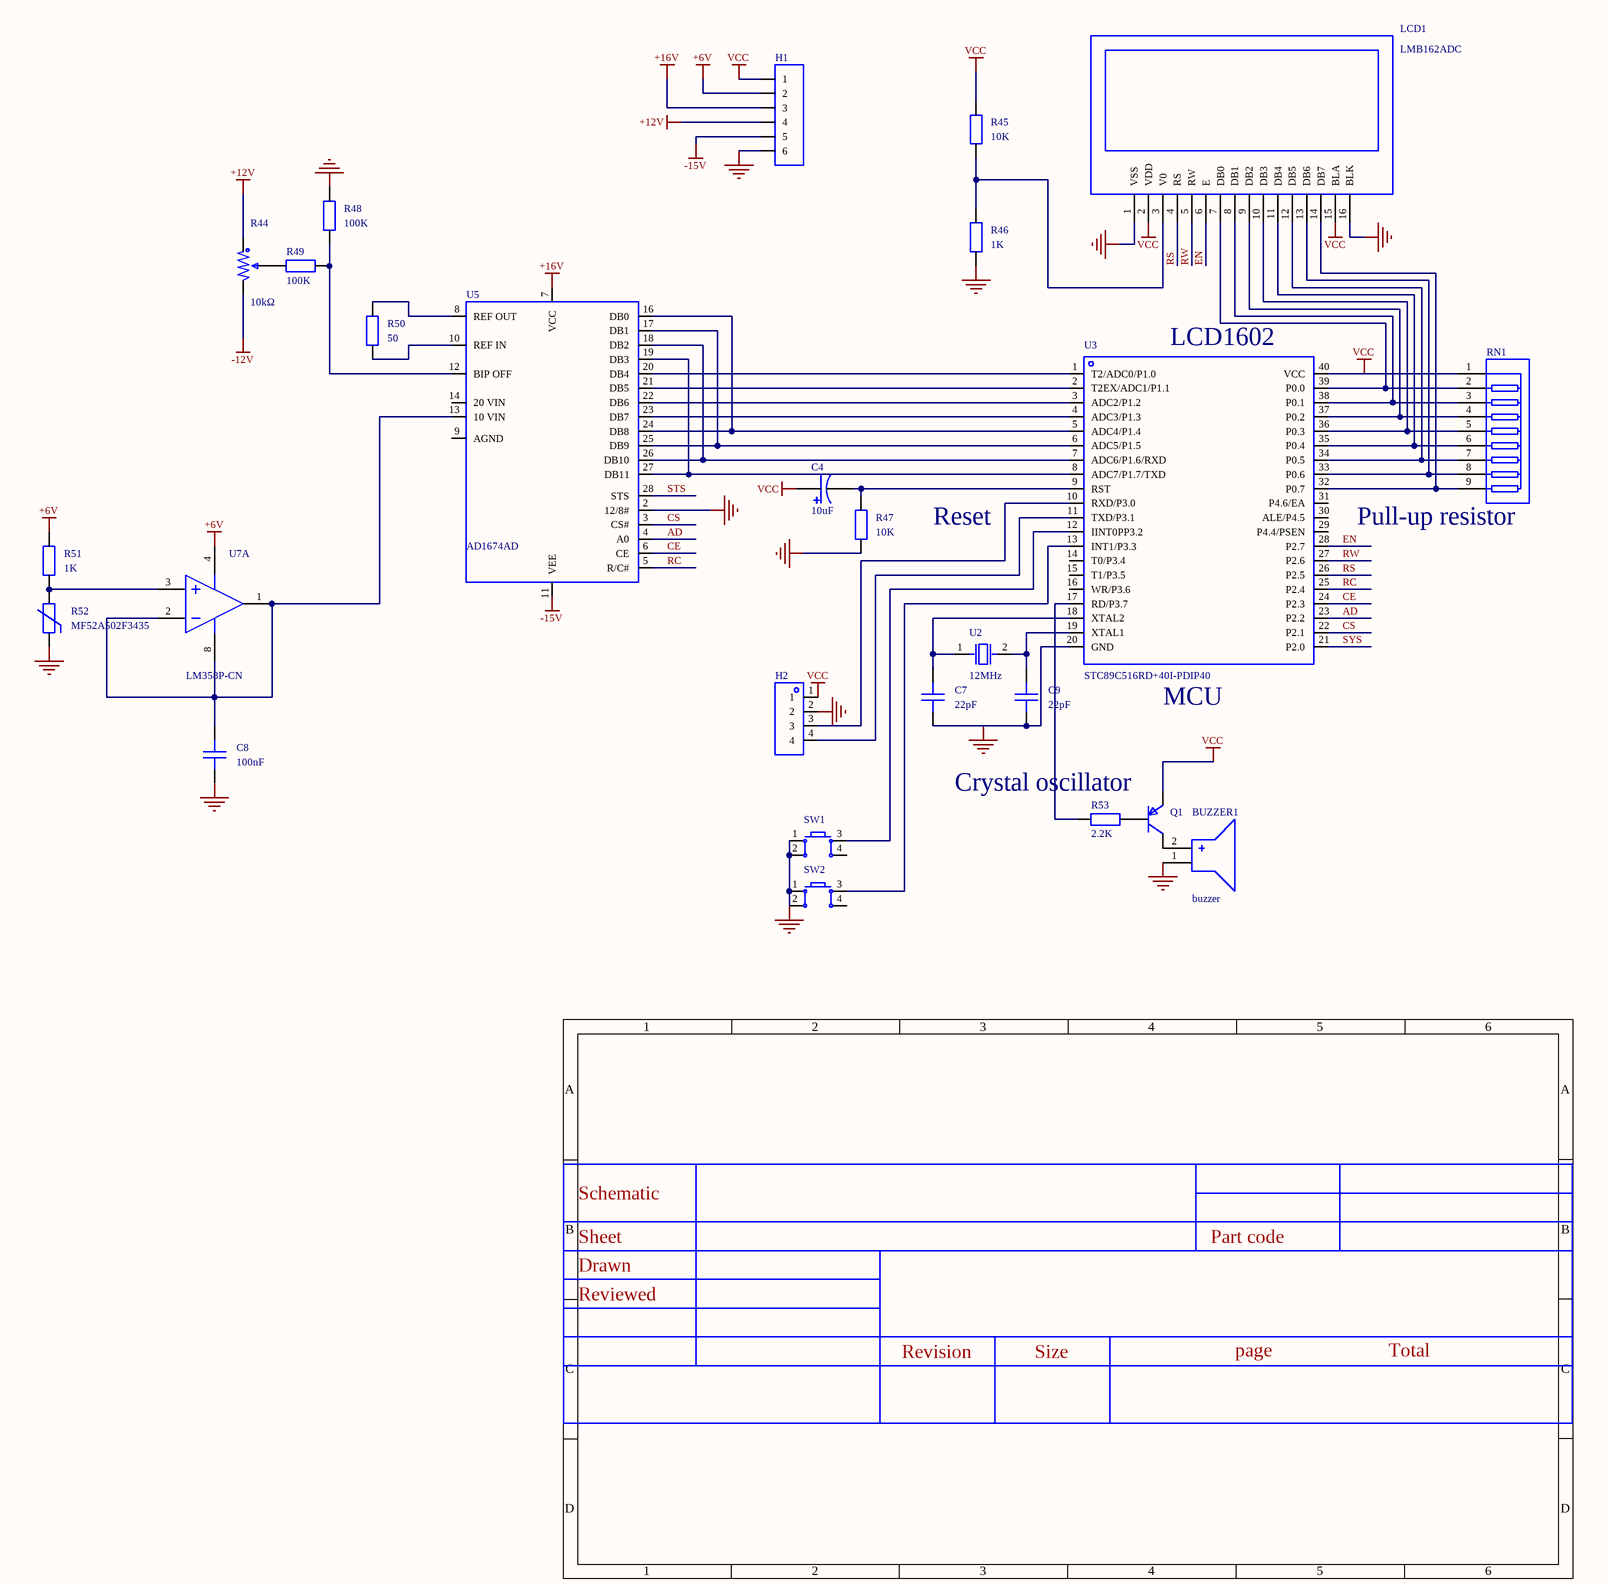
[diagram p0: MISC51839-3.schdoc]
# Altium project MISC51839-2.PrjPcb
1 sheet, 26 parts. Net scope: global (net labels, ports and power ports of the same name join across sheets).
Board file: MISC51839.pcbdoc

## Sheet MISC51839-3.schdoc
size 178 x 98 mm; Version: V1.0; @Project Name: MISC51839; @Page Count: 1; @Update Date: 2025-05-19; @Create Date: 2025-05-19; @Schematic Name: MISC51839; @Page No: 1; @Board Name: MISC51839; @Create Time: 08:04:37; @Update Time: 08:33:31

### Parts
BUZZER1  buzzer  [BUZ-TH_BD12.0-P6.00-D0.9-RD]
C4  10uF  [CAP-TH_BD6.3-P2.50-D1.0-FD]
C7  22pF  [C0603]
C8  100nF  [C0805]
C9  22pF  [C0603]
H1  (no value)  [HDR-TH_6P-P2.54-V-M-1]
H2  (no value)  [HDR-TH_4P-P2.54-V-F]
LCD1  LMB162ADC  [LCD1602]
Q1  (no value)  [S8550P_SOT]
R44  10kΩ  [RES-ADJ-SMD_RM065-V1]
R45  10K  [R0603]
R46  1K  [R0603]
R47  10K  [R0603]
R48  100K  [R0603]
R49  100K  [R0603]
R50  50  [R0603]
R51  1K  [R0603]
R52  MF52A502F3435  [RES-TH_BD2.0-P1.80-D0.3]
R53  2.2K  [R0603]
RN1  -  [RES-ARRAY-TH_9P-P2.54-D1.0]
SW1  (no value)  [SW-TH_4P-L6.0-W6.0-P4.50-LS6.5]
SW2  (no value)  [SW-TH_4P-L6.0-W6.0-P4.50-LS6.5]
U2  12MHz  [HC-49US_L11.0-W4.6-P4.88]
U3  STC89C516RD+40I-PDIP40  [DIP-40_L52.3-W13.9-P2.54-LS15.2-BL]
U5  AD1674AD  [CDIP-28_L35.5-W14.8-P2.54-LS15.3-BL]
U7  LM358P-CN  [SOIC-8_L5.0-W4.0-P1.27-LS6.0-BL]  (part A of 2)

### Nets
+6V: H1.2 R51.2 U7.4(V-)
+12V: H1.4 R44.1
+16V: H1.3 U5.7(VCC)
-12V: R44.3
-15V: H1.5 U5.11(VEE)
GND: BUZZER1.1(-) C7.1 C8.1 C9.1 H1.6 H2.2 LCD1.1(VSS) LCD1.16(BLK) R46.1 R47.1 R48.2 R52.1 SW1.1 SW1.2 SW2.1 SW2.2 U3.20(GND) U5.2(12/8#)
VCC: C4.1 H1.1 H2.1 LCD1.2(VDD) LCD1.15(BLA) Q1.2(E) R45.2 RN1.1 U3.40(VCC)
AD: U3.23(P2.2) U5.4(A0)
CE: U3.24(P2.3) U5.6(CE)
CS: U3.22(P2.1) U5.3(CS#)
EN: LCD1.6(E) U3.28(P2.7)
RC: U3.25(P2.4) U5.5(R/C#)
RS: LCD1.4(RS) U3.26(P2.5)
RW: LCD1.5(RW) U3.27(P2.6)
STS: U5.28(STS)
SYS: U3.21(P2.0)
NetBUZZER1_2: BUZZER1.2(+) Q1.3(C)
NetC4_2: C4.2 R47.2 U3.9(RST)
NetC7_2: C7.2 U2.1(OSC1) U3.18(XTAL2)
NetC8_2: C8.2 U5.13(10_VIN) U7.1(OUT1) U7.2(IN1-) U7.8(V+)
NetC9_2: C9.2 U2.2(OSC2) U3.19(XTAL1)
NetH2_3: H2.3 U3.10(RXD/P3.0)
NetH2_4: H2.4 U3.11(TXD/P3.1)
NetLCD1_3: LCD1.3(V0) R45.1 R46.2
NetLCD1_7: LCD1.7(DB0) RN1.2 U3.39(P0.0)
NetLCD1_8: LCD1.8(DB1) RN1.3 U3.38(P0.1)
NetLCD1_9: LCD1.9(DB2) RN1.4 U3.37(P0.2)
NetLCD1_10: LCD1.10(DB3) RN1.5 U3.36(P0.3)
NetLCD1_11: LCD1.11(DB4) RN1.6 U3.35(P0.4)
NetLCD1_12: LCD1.12(DB5) RN1.7 U3.34(P0.5)
NetLCD1_13: LCD1.13(DB6) RN1.8 U3.33(P0.6)
NetLCD1_14: LCD1.14(DB7) RN1.9 U3.32(P0.7)
NetQ1_1: Q1.1(B) R53.2
NetR44_2: R44.2 R49.2
NetR48_1: R48.1 R49.1 U5.12(BIP_OFF)
NetR50_1: R50.1 U5.10(REF_IN)
NetR50_2: R50.2 U5.8(REF_OUT)
NetR51_1: R51.1 R52.2 U7.3(IN1+)
NetR53_1: R53.1 U3.17(RD/P3.7)
NetSW1_3: SW1.3 U3.12(IINT0PP3.2)
NetSW2_3: SW2.3 U3.13(INT1/P3.3)
NetU3_1: U3.1(T2/ADC0/P1.0) U5.20(DB4)
NetU3_2: U3.2(T2EX/ADC1/P1.1) U5.21(DB5)
NetU3_3: U3.3(ADC2/P1.2) U5.22(DB6)
NetU3_4: U3.4(ADC3/P1.3) U5.23(DB7)
NetU3_5: U3.5(ADC4/P1.4) U5.16(DB0) U5.24(DB8)
NetU3_6: U3.6(ADC5/P1.5) U5.17(DB1) U5.25(DB9)
NetU3_7: U3.7(ADC6/P1.6/RXD) U5.18(DB2) U5.26(DB10)
NetU3_8: U3.8(ADC7/P1.7/TXD) U5.19(DB3) U5.27(DB11)

Not connected (* = marked no-connect by the designer): SW1 4; SW2 4; U3 14(T0/P3.4) 15(T1/P3.5) 16(WR/P3.6) 29(P4.4/PSEN) 30(ALE/P4.5) 31(P4.6/EA); U5 9(AGND) 14(20_VIN)

### Notes on the sheet
- (near U3) LCD1602
- Reset
- (near RN1) Pull-up resistor
- (near U3) MCU
- (near Q1) Crystal oscillator
- 2025-05-19
- Schematic
- Sheet
- Part code
- P1
- Reviewed
- Drawn
- Revision
- Size
- page
- Total
- A4
- 1

### Library data of the parts
BUZZER1 = buzzer: AddInBom: yes; ModelId: af17e4151ed84fc2a628230bf2376363; ModelTransform: 472.44,472.176,0,270,0,0,0,0,-196.85; Symbol: BUZZER; Device: buzzer; LCSC Part Name: buzzer; SupplierPart: C9900014030; ManufacturerPart: buzzer; Supplier Footprint: buzzer; Supplier: LCSC; ConvertToPcb: yes; FootprintName: BUZ-TH_BD12.0-P6.00-D0.9-RD; ModelName: BUZ-TH_BD12.0-P6.00-D0.9-RD
C4 = LKMC1202E100MF: Capacitance:10uF; Tolerance:±20%; Rated voltage:250V; Ripple current:-; Equivalent series resistance:-;; Manufacturer: Ymin(永铭); AddInBom: yes; ModelId: 0a4db4bf24b443b3be4905be97ff10c5; ModelTransform: 248.4247,247.99777,0,0,0,0,0,0,-137.795; Tolerance: ±20%; Rated Voltage: 250V; φD: 6.3mm; L: 12mm; Lifetime @ Temp: 9000hrs@105℃; Symbol: LKMC1202E100MF; Device: LKMC1202E100MF; LCSC Part Name: 10uF ±20% 250V; SupplierPart: C443243; ManufacturerPart: LKMC1202E100MF; Supplier Footprint: 插件,D6.3xL12mm; JLCPCB Part Class: Extended library; Datasheet: https://atta.szlcsc.com/upload/public/pdf/source/20200220/C487520_443A40905984A455D375EE990FEAA9E8.pdf; Supplier: LCSC; ConvertToPcb: yes; FootprintName: CAP-TH_BD6.3-P2.50-D1.0-FD; ModelName: CAP-TH_BD6.3-P2.50-D1.0-FD; Value: 10uF; Ripple Current: -; Equivalent Series Resistance(ESR): -; Lead Spacing: 2.5mm
C7 C9 = CAP_0603: ConvertToPcb: yes; SymbolName: CapAcitance; ModelId: ac125912035d415993ca9572d50418b1; ModelName: C0603_L1.6-W0.8-H0.8; ModelTransform: 62.992,31.496,0,0,0,0,0,0,0; Value: 22pF; Device: CAP_0603; AddInBom: yes; Supplier Footprint: 0603; FootprintName: C0603
C8 = CAP_0805: ConvertToPcb: yes; SymbolName: CapAcitance; ModelId: 1ba041120af144c991958decab20d241; ModelName: C0805_L2.0-W1.3-H1.3; ModelTransform: 78.74,51.181,0,0,0,0,0,0.0005,0; Device: CAP_0805; AddInBom: yes; Supplier Footprint: 0805; FootprintName: C0805; Value: 100nF
H1 = HDR-M_2.54_1x6P: Symbol: Header-Male-2.54_1x6; ConvertToPcb: yes; ModelId: 60739dffc9b04830a286435b0fefbd4a; ModelName: HDR2.54-M-LI-1X6P; ModelTransform: 599.999,100,0,0,0,0,0,0,-118.11; Device: HDR-M_2.54_1x6P; AddInBom: yes; SupplierPart: C37208; Supplier Footprint: 插件; FootprintName: HDR-TH_6P-P2.54-V-M-1
H2 = HDR-F_2.54_1x4P: Symbol: 2.54-1*4P female; ConvertToPcb: yes; ModelId: d187812051054f85879fcaa51a310d8e; ModelTransform: 419.6842,98.464,0,0,0,0,0,0,-118.11; Device: HDR-F_2.54_1x4P; AddInBom: yes; SupplierPart: C2718488; Supplier Footprint: 插件; FootprintName: HDR-TH_4P-P2.54-V-F; ModelName: HDR-TH_4P-P2.54-V-F
LCD1 = LMB162ADC: 16x2 character LCD module; AddInBom: yes; ModelId: f9d832f46a914cadb50fc4d4cefd2517; ModelTransform: 3149.6,1417.32,0,0,0,0,0,0,-118.11; Symbol: LMB162ADC; Device: LMB162ADC; LCSC Part Name: LMB162ADC; SupplierPart: C9741; ManufacturerPart: LMB162ADC; Supplier Footprint: SIP; JLCPCB Part Class: Extended library; Supplier: LCSC; ConvertToPcb: yes; FootprintName: LCD1602; ModelName: LCD1602
Q1 = S8550_SOT_PNP: Symbol: PNP; ConvertToPcb: yes; ModelId: 9c0df02d6f3e44e889da37f3e5bf5496; ModelName: SOT-23-3_L2.9-W1.4-P1.90-LS2.5-BR; ModelTransform: 98.43,114.17,37.91,0,0,0,0,0,0; Device: S8550_SOT_PNP; AddInBom: yes; Supplier Footprint: SOT-23; FootprintName: S8550P_SOT
R44 = RM065-103(10K): Resistance:10kΩ; Tolerance:±25%; Power:100mW;; Manufacturer: BOCHEN(博晨); AddInBom: yes; ModelId: c816c2b7942147f5a832150e8ef6960c; ModelTransform: 255.905,283.464,0,0,0,0,0.025,-3.937,-157.48; Tolerance: ±25%; Power(Watts): 100mW; Symbol: RM065-103(10K); Device: RM065-103(10K); LCSC Part Name: 10kΩ ±25%; SupplierPart: C5205021; ManufacturerPart: RM065-103(10K); Supplier Footprint: 插件; JLCPCB Part Class: Extended Part; Datasheet: https://atta.szlcsc.com/upload/public/pdf/source/20221019/6263C46FBC7F1B66CBAADA74DC5EFAA2.pdf; Supplier: LCSC; ConvertToPcb: yes; FootprintName: RES-ADJ-SMD_RM065-V1; ModelName: RES-ADJ-SMD_RM065-V1; Value: 10kΩ
R45-R51 R53 = Res_0603: Symbol: Resistor; ConvertToPcb: yes; ModelId: fc143cca1e79419f9cd78b61e9279f08; ModelTransform: 31.8897,63.7794,0,90,0,0,0,0,0; Device: Res_0603; AddInBom: yes; Supplier Footprint: 0603; FootprintName: R0603; ModelName: R0603
  R45 R47: Value: 10K
  R46 R51: Value: 1K
  R48 R49: Value: 100K
  R50: Value: 50
  R53: Value: 2.2K
R52 = MF52A502F3435: Resistance:5kΩ; B value (25℃/50℃):3435K; B value tolerance:±1%;; Manufacturer: SURGING(绍鑫); AddInBom: yes; ModelId: c3233c37e82b4c54ae488fe02709f9ae; ModelTransform: 86.58227,86.38046,0,0,0,0,-0.002,0,-157.48; Resistance @ 25℃: 5kΩ; B Constant (25℃/50℃): 3435K; B Constant Tolerance: ±1%; Symbol: MF52A502F3435; Device: MF52A502F3435; LCSC Part Name: MF52A502F3435; SupplierPart: C5439705; ManufacturerPart: MF52A502F3435; Supplier Footprint: -; Supplier: LCSC; ConvertToPcb: yes; FootprintName: RES-TH_BD2.0-P1.80-D0.3; ModelName: RES-TH_BD2.0-P1.80-D0.3
RN1 = 排阻 10 K 5%: Number of resistors:-; Resistance:-; Power per element:-;; Symbol: 10 K 5%; Device: Resistor network 10 K 5%; AddInBom: yes; ModelId: d106c67f29e14d8080ba548247a719a1; ModelName: SIP-9_L22.8-W3.0-H8.5-P2.54; ModelTransform: 917.49722,118.11,0,0,0,0,0,0,-137.795; LCSC Part Name: 10KΩ (103) ±5%; SupplierPart: C26615; ManufacturerPart: 排阻 10 K 5%; Supplier Footprint: 插件; JLCPCB Part Class: Extended library; Supplier: LCSC; ConvertToPcb: yes; FootprintName: RES-ARRAY-TH_9P-P2.54-D1.0; Number of Resistors: -; Value: -; Power(Watts): -; Number of Pins: -
SW1 SW2 = Key_TH_6x6x6: 触点电流:50mA;额定电压(DC):12V;绝缘电阻:100MΩ;电路结构:单刀单掷;安装方式:直插;按钮形状:圆形按钮;按钮/盖帽颜色:黑色;作用力:260gf@±30gf;工作温度:-25℃~+70℃;引脚样式:PC引脚;开关长度:6mm;开关宽度:6mm;开关高度:6mm;带支架:否;; Symbol: Tactile switch; ConvertToPcb: yes; ModelId: 20eee248bc684ccd8cbdbb1d0d91ec6f; ModelName: SW-TH_4P-L6.0-W6.0-H5.0-LS6.5-P4.50; ModelTransform: 236.22,323.03,0,90,0,0,0,0,-137.795; Device: Key_TH_6x6x6; AddInBom: yes; SupplierPart: C2837516; Supplier Footprint: 插件; FootprintName: SW-TH_4P-L6.0-W6.0-P4.50-LS6.5
U2 = ECS-120-S-4: Frequency:12MHz; Room-temperature frequency tolerance:±30ppm; External load capacitance:-; Frequency stability (full temperature):±50ppm;; Manufacturer: ECS; AddInBom: yes; ModelId: 59d05c800eee432cb051aa4925461fda; ModelName: HC-49US_L11.0-W4.7-H3.5-P4.88; ModelTransform: 432.44473,183.0705,0,0,0,0,0,0,-137.795; Normal temperature Frequency Tolerance: ±30ppm; Frequency Stability(Full temperature range): ±50ppm; Equivalent Series Resistance (ESR): 60Ω; Symbol: ECS-120-S-4; Device: ECS-120-S-4; LCSC Part Name: 12MHz ±30ppm; ManufacturerPart: ECS-120-S-4; Supplier Footprint: HC-49S; JLCPCB Part Class: Extended library; Datasheet: https://atta.szlcsc.com/upload/public/pdf/source/20210402/81F084B668D60DFAE850A61100CCABAF.pdf; Supplier: LCSC; ConvertToPcb: yes; FootprintName: HC-49US_L11.0-W4.6-P4.88; Value: 12MHz; External load capacitor: -; Operating Temperature: -10℃~+70℃
U3 = STC89C516RD+40I-PDIP40: CPU core:51 series; Program storage capacity:61KB; Total RAM:1.25KB; GPIO port count:35; Operating voltage range:3.5V~5.5V; CPU max clock:-; Program memory type:FLASH;; Manufacturer: STC(宏晶); AddInBom: yes; ModelId: 16d4686a009b4ddca948f91eddb57b14; ModelName: DIP-40_L52.3-W13.8-H4.0-LS15.24-P2.54; ModelTransform: 2059.051,615.743,0,0,0,0,0,0,-129.921; Program Storage Size: 61KB; RAM Size: 1.25KB; GPIO Ports Number: 35; Program Memory Type: FLASH; 16Bit Timer: 3; UART/USART: 1; Peripheral/Function: Watchdog; Symbol: STC89C516RD+40I-PDIP40; Device: STC89C516RD+40I-PDIP40; LCSC Part Name: STC89C516RD+40I-PDIP40; SupplierPart: C52225; ManufacturerPart: STC89C516RD+40I-PDIP40; Supplier Footprint: DIP-40; JLCPCB Part Class: Extended library; Datasheet: https://atta.szlcsc.com/upload/public/pdf/source/20180614/C87831_BBAF7FB8B286C29ACE4E9B180C033FEC.pdf; Supplier: LCSC; ConvertToPcb: yes; FootprintName: DIP-40_L52.3-W13.9-P2.54-LS15.2-BL; CPU Core: 51 series; Operating Voltage Range: 3.5V~5.5V; CPU Maximum Speed: -; Operating Temperature Range: -40℃~+85℃; ADC (Bit): -; DAC (Bit): -; PWM (Bit): -; 8Bit Timer: -; 32Bit Timer: -; CAN: -; I2C: -; I2S: -; SPI: -; Universal Serial Bus: -; Internal Comparator: -; communication protocol: -; Watchdog: Yes; Real-Time Clock: -; Infrared Data Association: -; Low-Voltage Detect: -; CCP Capture/Compare: -; Secure Digital Input and Output: -; Direct Memory Access: -; Internal Oscillator: -
U5 = AD1674AD: Interface:Parallel; Supply voltage:11.4V~16.5V; Sampling rate:100kHz; Resolution:12 bit;; Manufacturer: ADI(亚德诺); AddInBom: yes; number of channels: 1; sampling frequency: 100kHz; resolution: 12 bit; ModelId: 35b7b3e94b8241fb9aab19a88eb4728c; ModelTransform: 1489.46734,598.424,0,0,0,0,0,0,-177.165; Symbol: AD1674AD; Device: AD1674AD; LCSC Part Name: AD1674AD; SupplierPart: C706707; ManufacturerPart: AD1674AD; Supplier Footprint: CDIP-28; JLCPCB Part Class: Extended library; Datasheet: https://atta.szlcsc.com/upload/public/pdf/source/20220519/7875144D47F22D938E794B4CB59411AD.pdf; Supplier: LCSC; ConvertToPcb: yes; Interface: Parallel; Supply Voltage: 11.4V~16.5V; Operating Temperature: -40℃~+85℃; FootprintName: CDIP-28_L35.5-W14.8-P2.54-LS15.3-BL; ModelName: CDIP-28_L35.5-W14.8-P2.54-LS15.3-BL
U7 = LM358P-CN: Manufacturer: ChipNobo(无边界); Relevance: []; AddInBom: yes; ModelId: 5dc2af053da0476fab11ee64b9a10a94; ModelName: PDIP-8_L9.6-W6.4-P2.54-LS7.62-BL; ModelTransform: 377.952,309.842,0,0,0,0,0,0,-137.795; Symbol: LM358P-CN; Device: LM358P-CN; LCSC Part Name: LM358P-CN; SupplierPart: C42436861; ManufacturerPart: LM358P-CN; Supplier Footprint: DIP-8; Datasheet: https://atta.szlcsc.com/upload/public/pdf/source/20250107/42CF9E225B98BCF3AB4ADCCD694C1100.pdf; Supplier: LCSC; ConvertToPcb: yes; FootprintName: SOIC-8_L5.0-W4.0-P1.27-LS6.0-BL